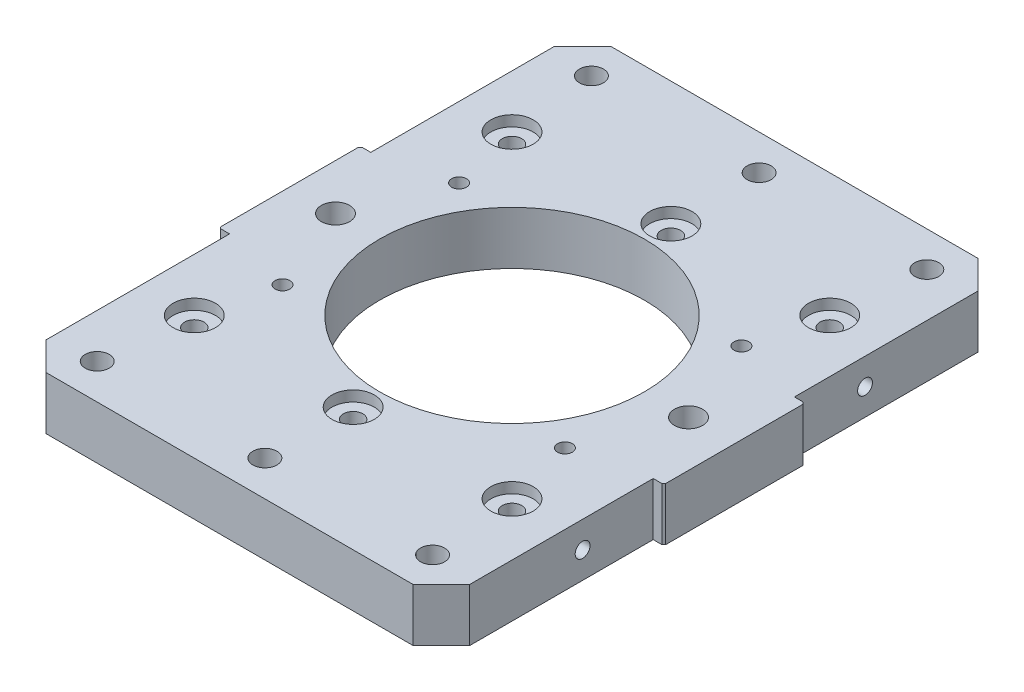
from build123d import *

# Parameters (mm, degrees)
SKETCH1_W                  = 120
SKETCH1_H                  = 160
BOSS_EXTRUDE1_DEPTH        = 15
CHAMFER1_SIZE              = 8
SKETCH2_R                  = 37.5
CUT_EXTRUDE1_DEPTH         = 23
SKETCH3_R                  = 1
CUT_EXTRUDE2_DEPTH         = 10
M5_TAPPED_HOLE1_D          = 4.2
SKETCH8_R                  = 3
CUT_EXTRUDE4_DEPTH         = 55
M8_TAPPED_HOLE1_D          = 6.8
SKETCH11_R                 = 2.5
CUT_EXTRUDE5_DEPTH         = 33
SKETCH12_R                 = 4
CUT_EXTRUDE6_DEPTH         = 6
SKETCH13_W                 = 3
SKETCH13_H                 = 40
BOSS_EXTRUDE2_DEPTH        = 15
CHAMFER2_SIZE              = 0.5
SKETCH14_R                 = 1.794169989
SKETCH14_R_2               = 1.756446965
CUT_EXTRUDE7_DEPTH         = 5
M5_TAPPED_HOLE2_AT_2_COUNT = 2
M5_TAPPED_HOLE2_AT_2_PITCH = 80
SKETCH16_R                 = 2.75
CUT_EXTRUDE8_DEPTH         = 55
SKETCH17_R                 = 6
CUT_EXTRUDE9_DEPTH         = 3


with BuildPart() as part:
    # Sketch1 → Boss-Extrude1 (new body)
    with BuildSketch(Plane(origin=(0, 0, 0), x_dir=(1, 0, 0), z_dir=(0, 1, 0))):
        Rectangle(SKETCH1_W, SKETCH1_H)
    extrude(amount=BOSS_EXTRUDE1_DEPTH)

    # Chamfer1
    chamfer1_edges = [part.edges().sort_by_distance(p)[0] for p in [
        (60, 7.5, 80),
        (-60, 7.5, 80),
        (-60, 7.5, -80),
        (60, 7.5, -80),
    ]]
    chamfer(chamfer1_edges, length=CHAMFER1_SIZE)

    # Sketch2 → Cut-Extrude1 (cut)
    with BuildSketch(Plane(origin=(0, 15, 0), x_dir=(1, 0, 0), z_dir=(0, 1, 0))):
        with Locations(Location((0, 0, 0), (0, 0, 270))):
            Circle(SKETCH2_R)
    extrude(amount=-CUT_EXTRUDE1_DEPTH, mode=Mode.SUBTRACT)

    # Sketch3 → Cut-Extrude2 (cut)
    with BuildSketch(Plane.XZ):
        with Locations(Location((-40, 25, 0), (0, 0, 270))):
            Circle(SKETCH3_R)
        with Locations(Location((40, 25, 0), (0, 0, 90))):
            Circle(SKETCH3_R)
        with Locations(Location((-40, -25, 0), (0, 0, 90))):
            Circle(SKETCH3_R)
        with Locations(Location((40, -25, 0), (0, 0, 270))):
            Circle(SKETCH3_R)
    extrude(amount=-CUT_EXTRUDE2_DEPTH, mode=Mode.SUBTRACT)

    # M5 Tapped Hole1 (through all)
    with Locations(Plane(origin=(-40, 0, 25), x_dir=(0, 0, -1), z_dir=(0, -1, 0))):
        with Locations((0, 0), (0, 80), (50, 80), (50, 0)):
            Hole(M5_TAPPED_HOLE1_D / 2)

    # Sketch8 → Cut-Extrude4 (cut)
    with BuildSketch(Plane.XZ):
        with Locations(Location((-47.5, 70, 0), (0, 0, 270))):
            Circle(SKETCH8_R)
        with Locations(Location((0, 70, 0), (0, 0, 270))):
            Circle(SKETCH8_R)
        with Locations(Location((47.5, 70, 0), (0, 0, 90))):
            Circle(SKETCH8_R)
        with Locations(Location((47.5, -70, 0), (0, 0, 270))):
            Circle(SKETCH8_R)
        with Locations(Location((0, -70, 0), (0, 0, 90))):
            Circle(SKETCH8_R)
        with Locations(Location((-47.5, -70, 0), (0, 0, 90))):
            Circle(SKETCH8_R)
    extrude(amount=-CUT_EXTRUDE4_DEPTH, mode=Mode.SUBTRACT)

    # M8 Tapped Hole1 (through all)
    with Locations(Plane(origin=(47.5, 0, -70), x_dir=(0, 0, -1), z_dir=(0, -1, 0))):
        with Locations((0, 0), (0, -47.5), (0, -95), (-140, -95), (-140, -47.5), (-140, 0)):
            Hole(M8_TAPPED_HOLE1_D / 2)

    # Sketch11 → Cut-Extrude5 (cut)
    with BuildSketch(Plane.XZ):
        with Locations(Location((-50, 0, 0), (0, 0, 270))):
            Circle(SKETCH11_R)
        with Locations(Location((50, 0, 0), (0, 0, 90))):
            Circle(SKETCH11_R)
    extrude(amount=-CUT_EXTRUDE5_DEPTH, mode=Mode.SUBTRACT)

    # Sketch12 → Cut-Extrude6 (cut)
    with BuildSketch(Plane(origin=(0, 15, 0), x_dir=(1, 0, 0), z_dir=(0, 1, 0))):
        with Locations(Location((-50, 0, 0), (0, 0, 270))):
            Circle(SKETCH12_R)
        with Locations(Location((50, 0, 0), (0, 0, 270))):
            Circle(SKETCH12_R)
    extrude(amount=-CUT_EXTRUDE6_DEPTH, mode=Mode.SUBTRACT)

    # Sketch13 → Boss-Extrude2 (add)
    with BuildSketch(Plane(origin=(0, 15, 0), x_dir=(1, 0, 0), z_dir=(0, 1, 0))):
        with Locations((-61.5, 0)):
            Rectangle(SKETCH13_W, SKETCH13_H)
        with Locations((61.5, 0)):
            Rectangle(SKETCH13_W, SKETCH13_H)
    extrude(amount=-BOSS_EXTRUDE2_DEPTH)

    # Chamfer2
    chamfer2_edges = [part.edges().sort_by_distance(p)[0] for p in [
        (63, 7.5, -20),
        (63, 7.5, 20),
        (-63, 7.5, -20),
        (-63, 7.5, 20),
    ]]
    chamfer(chamfer2_edges, length=CHAMFER2_SIZE)

    # Sketch14 → Cut-Extrude7 (cut)
    with BuildSketch(Plane(origin=(60, 0, 0), x_dir=(0, 0, -1), z_dir=(1, 0, 0))):
        with Locations((-40, 7.5)):
            Circle(SKETCH14_R)
        with Locations((40, 7.5)):
            Circle(SKETCH14_R_2)
    extrude(amount=-CUT_EXTRUDE7_DEPTH, mode=Mode.SUBTRACT)

    # Sketch15 → M5 Tapped Hole2 (revolve, cut)
    with BuildSketch(Plane(origin=(60, 7.5, 40), x_dir=(0, 0, -1), z_dir=(0, 1, 0))):
        Polygon((0, 0), (0, 13.6618073), (2.1, 12.4), (2.1, 0), align=None)
    m5_tapped_hole2 = revolve(axis=Axis((66.35, 7.5, 40), (-1, 0, 0)), mode=Mode.SUBTRACT)

    # M5 Tapped Hole2 at 2: M5 Tapped Hole2 ×2
    with Locations(*[(0, 0, -i * M5_TAPPED_HOLE2_AT_2_PITCH) for i in range(1, M5_TAPPED_HOLE2_AT_2_COUNT)]):
        add(m5_tapped_hole2, mode=Mode.SUBTRACT)

    # Mirror1: M5 Tapped Hole2 across plane
    add(m5_tapped_hole2.mirror(Plane(origin=(0, 0, 0), x_dir=(0, 0, 1), z_dir=(1, 0, 0))), mode=Mode.SUBTRACT)

    # Mirror1 copy 1 sketch → Mirror1 copy 1 (revolve, cut)
    with BuildSketch(Plane(origin=(-60, 7.5, -40), x_dir=(0, 0, -1), z_dir=(0, 1, 0))):
        Polygon((0, 0), (0, -13.6618073), (2.1, -12.4), (2.1, 0), align=None)
    revolve(axis=Axis((-66.35, 7.5, -40), (-1, 0, 0)), mode=Mode.SUBTRACT)

    # Sketch16 → Cut-Extrude8 (cut)
    with BuildSketch(Plane(origin=(0, 15, 0), x_dir=(1, 0, 0), z_dir=(0, 1, 0))):
        with Locations(Location((0, 45, 0), (0, 0, 270))):
            Circle(SKETCH16_R)
        with Locations(Location((45, 45, 0), (0, 0, 270))):
            Circle(SKETCH16_R)
        with Locations(Location((-45, 45, 0), (0, 0, 270))):
            Circle(SKETCH16_R)
        with Locations(Location((-45, -45, 0), (0, 0, 270))):
            Circle(SKETCH16_R)
        with Locations(Location((45, -45, 0), (0, 0, 270))):
            Circle(SKETCH16_R)
        with Locations(Location((0, -45, 0), (0, 0, 270))):
            Circle(SKETCH16_R)
    extrude(amount=-CUT_EXTRUDE8_DEPTH, mode=Mode.SUBTRACT)

    # Sketch17 → Cut-Extrude9 (cut)
    with BuildSketch(Plane(origin=(0, 15, 0), x_dir=(1, 0, 0), z_dir=(0, 1, 0))):
        with Locations(Location((-45, -45, 0), (0, 0, 270))):
            Circle(SKETCH17_R)
        with Locations(Location((0, -45, 0), (0, 0, 270))):
            Circle(SKETCH17_R)
        with Locations(Location((45, -45, 0), (0, 0, 270))):
            Circle(SKETCH17_R)
        with Locations(Location((0, 45, 0), (0, 0, 270))):
            Circle(SKETCH17_R)
        with Locations(Location((45, 45, 0), (0, 0, 270))):
            Circle(SKETCH17_R)
        with Locations(Location((-45, 45, 0), (0, 0, 270))):
            Circle(SKETCH17_R)
    extrude(amount=-CUT_EXTRUDE9_DEPTH, mode=Mode.SUBTRACT)


solid = part.part
